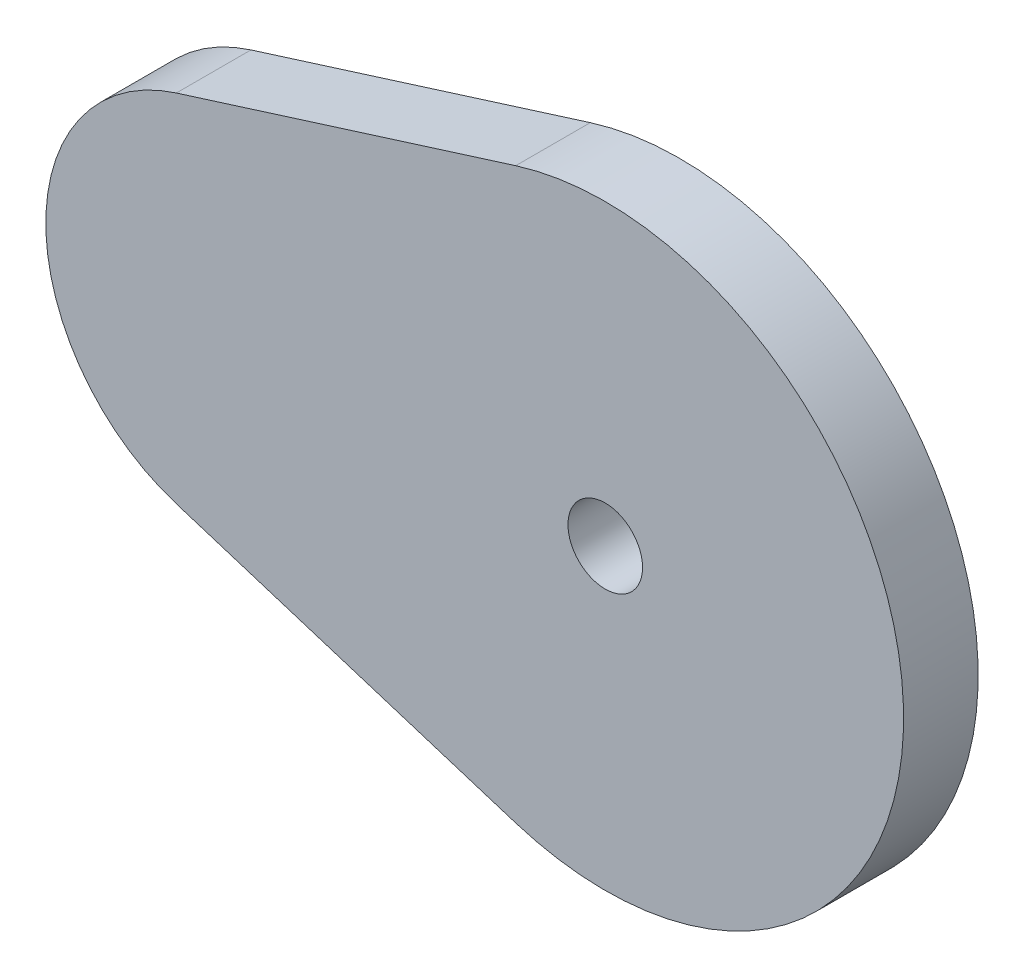
from build123d import *

# Parameters (mm, degrees)
SKETCH1_R           = 5
BOSS_EXTRUDE1_DEPTH = 10


with BuildPart() as part:
    # Sketch1 → Boss-Extrude1 (new body)
    with BuildSketch(Plane.XY):
        with BuildLine():
            Line((-57.5, 23.848480035), (-12, 38.157568057))
            ThreePointArc((-12, 38.157568057), (40, 0), (-12, -38.157568057))
            Line((-12, -38.157568057), (-57.5, -23.848480035))
            ThreePointArc((-57.5, -23.848480035), (-75, 0), (-57.5, 23.848480035))
        make_face()
        Circle(SKETCH1_R, mode=Mode.SUBTRACT)
    extrude(amount=BOSS_EXTRUDE1_DEPTH)


solid = part.part
